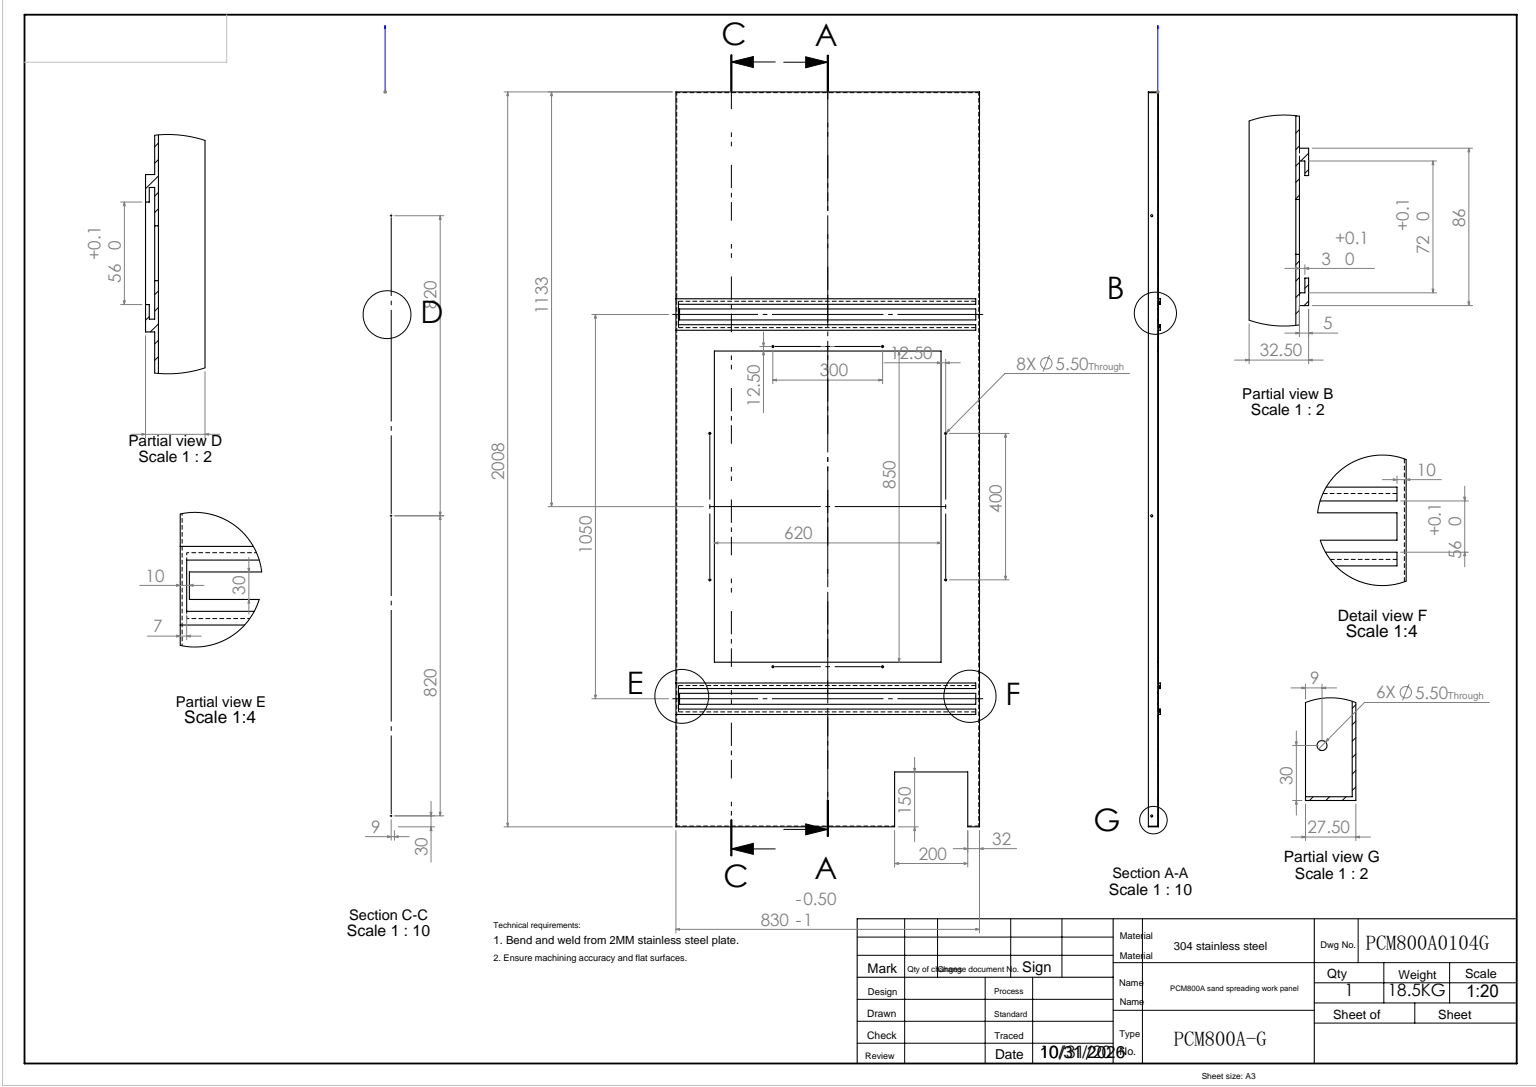
from build123d import *

# Parameters (mm, degrees)
SKETCH_1_W             = 830
SKETCH_1_H             = 2008
SKETCH_1_W_2           = 620
SKETCH_1_H_2           = 850
EXTRUDE_1_DEPTH        = 2
SKETCH_2_W             = 810
SKETCH_2_H             = 30
CUT_EXTRUDE_1_DEPTH    = 2
SKETCH_3_W             = 2
SKETCH_3_H             = 2008
EXTRUDE_2_DEPTH        = 25.5
SKETCH_4_W             = 200
SKETCH_4_H             = 150
CUT_EXTRUDE_2_DEPTH    = 2173.927575875
SKETCH_5_W             = 30
SKETCH_5_H             = 2
SKETCH_5_W_2           = 596
SKETCH_5_W_3           = 826
EXTRUDE_3_DEPTH        = 25.5
EXTRUDE_4_DEPTH        = 5
SKETCH_8_W             = 3
SKETCH_8_H             = 8
CUT_EXTRUDE_3_DEPTH    = 813
PATTERN_LINEAR_1_COUNT = 2
PATTERN_LINEAR_1_PITCH = 1050
SKETCH_9_R             = 2.75
CUT_EXTRUDE_4_DEPTH    = 126
SKETCH_10_R            = 2.75
CUT_EXTRUDE_5_DEPTH    = 1163


with BuildPart() as part:
    # 草图1 → 凸台-拉伸1 (new body)
    with BuildSketch(Plane.XY):
        with Locations((415, -1004)):
            Rectangle(SKETCH_1_W, SKETCH_1_H)
        with Locations((415, -1133)):
            Rectangle(SKETCH_1_W_2, SKETCH_1_H_2, mode=Mode.SUBTRACT)
    extrude(amount=EXTRUDE_1_DEPTH)

    # 草图2 → 切除-拉伸1 (cut)
    with BuildSketch(Plane.XY.offset(2)):
        with Locations((415, -1658)):
            Rectangle(SKETCH_2_W, SKETCH_2_H)
        with Locations((415, -608)):
            Rectangle(SKETCH_2_W, SKETCH_2_H)
    extrude(amount=-CUT_EXTRUDE_1_DEPTH, mode=Mode.SUBTRACT)

    # 草图3 → 凸台-拉伸2 (add)
    with BuildSketch(Plane.XY):
        with Locations((1, -1004)):
            Rectangle(SKETCH_3_W, SKETCH_3_H)
        with Locations((829, -1004)):
            Rectangle(SKETCH_3_W, SKETCH_3_H)
    extrude(amount=-EXTRUDE_2_DEPTH)

    # 草图4 → 切除-拉伸2 (cut, through all)
    with BuildSketch(Plane(origin=(0, 0, 0), x_dir=(-1, 0, 0), z_dir=(0, 0, -1))):
        with Locations((-698, -1933)):
            Rectangle(SKETCH_4_W, SKETCH_4_H)
    extrude(amount=-CUT_EXTRUDE_2_DEPTH, mode=Mode.SUBTRACT)

    # 草图5 → 凸台-拉伸3 (add)
    with BuildSketch(Plane(origin=(0, 0, 0), x_dir=(-1, 0, 0), z_dir=(0, 0, -1))):
        with Locations((-813, -2007)):
            Rectangle(SKETCH_5_W, SKETCH_5_H)
        with Locations((-300, -2007)):
            Rectangle(SKETCH_5_W_2, SKETCH_5_H)
        with Locations((-415, -1)):
            Rectangle(SKETCH_5_W_3, SKETCH_5_H)
    extrude(amount=EXTRUDE_3_DEPTH)

    # 草图7 → 凸台-拉伸4 (add)
    with BuildSketch(Plane.XY.offset(2)):
        Polygon((820, -564.997302091), (820, -580), (7, -580), (7, -636), (820, -636), (820, -651), (0, -651), (0, -564.997302091), align=None)
    extrude_4 = extrude(amount=EXTRUDE_4_DEPTH)

    # 草图8 → 切除-拉伸3 (cut)
    with BuildSketch(Plane(origin=(820, 0, 0), x_dir=(0, 0, -1), z_dir=(1, 0, 0))):
        with Locations((-3.5, -576)):
            Rectangle(SKETCH_8_W, SKETCH_8_H)
        with Locations((-3.5, -640)):
            Rectangle(SKETCH_8_W, SKETCH_8_H)
    cut_extrude_3 = extrude(amount=-CUT_EXTRUDE_3_DEPTH, mode=Mode.SUBTRACT)

    # 阵列(线性)1: 凸台-拉伸4, 切除-拉伸3 ×2
    with Locations(*[(0, -i * PATTERN_LINEAR_1_PITCH, 0) for i in range(1, PATTERN_LINEAR_1_COUNT)]):
        add(extrude_4)
        add(cut_extrude_3, mode=Mode.SUBTRACT)

    # 草图9 → 切除-拉伸4 (cut)
    with BuildSketch(Plane(origin=(0, 0, 0), x_dir=(-1, 0, 0), z_dir=(0, 0, -1))):
        with Locations((-565, -695.5)):
            Circle(SKETCH_9_R)
        with Locations((-265, -695.5)):
            Circle(SKETCH_9_R)
        with Locations((-737.5, -933)):
            Circle(SKETCH_9_R)
        with Locations((-737.5, -1333)):
            Circle(SKETCH_9_R)
        with Locations((-565, -1570.5)):
            Circle(SKETCH_9_R)
        with Locations((-265, -1570.5)):
            Circle(SKETCH_9_R)
        with Locations((-92.5, -1333)):
            Circle(SKETCH_9_R)
        with Locations((-92.5, -933)):
            Circle(SKETCH_9_R)
    extrude(amount=-CUT_EXTRUDE_4_DEPTH, mode=Mode.SUBTRACT)

    # 草图10 → 切除-拉伸5 (cut)
    with BuildSketch(Plane.ZY):
        with Locations(Location((-16.5, -1978, 0), (0, 0, 270))):
            Circle(SKETCH_10_R)
        with Locations(Location((-16.5, -1158, 0), (0, 0, 270))):
            Circle(SKETCH_10_R)
        with Locations(Location((-16.5, -338, 0), (0, 0, 270))):
            Circle(SKETCH_10_R)
    extrude(amount=-CUT_EXTRUDE_5_DEPTH, mode=Mode.SUBTRACT)


solid = part.part
